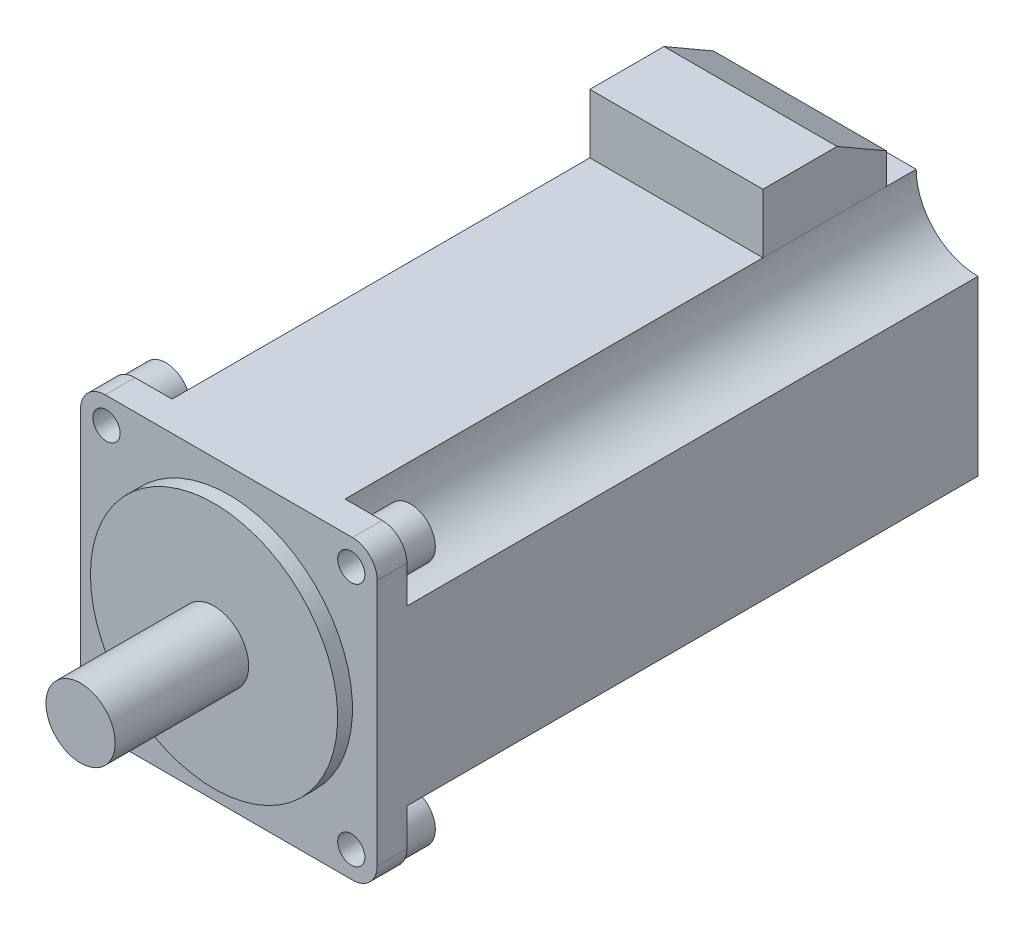
from build123d import *

# Parameters (mm, degrees)
SKETCH1_R                      = 7
BOSS_EXTRUDE1_DEPTH            = 30
SKETCH2_R                      = 25
BOSS_EXTRUDE2_DEPTH            = 3
SKETCH3_W                      = 60
SKETCH3_H                      = 60
BOSS_EXTRUDE3_DEPTH            = 6
BOSS_EXTRUDE4_DEPTH            = 115.5
SKETCH5_W                      = 35
SKETCH5_H                      = 25
BOSS_EXTRUDE5_DEPTH            = 12
CHAMFER1_SIZE                  = 10
CHAMFER1_SIZE2                 = 5.773502692
F_5_5_5_5_DIAMETER_HOLE1_D     = 5.5
F_5_5_5_5_DIAMETER_HOLE1_DEPTH = 20
F_5_5_5_5_DIAMETER_HOLE1_TIP   = 1.652366702
FILLET1_R                      = 5
SKETCH8_R                      = 5
BOSS_EXTRUDE6_DEPTH            = 6


with BuildPart() as part:
    # Sketch1 → Boss-Extrude1 (new body)
    with BuildSketch(Plane.XY):
        Circle(SKETCH1_R)
    extrude(amount=-BOSS_EXTRUDE1_DEPTH)

    # Sketch2 → Boss-Extrude2 (add)
    with BuildSketch(Plane(origin=(0, 0, -30), x_dir=(-1, 0, 0), z_dir=(0, 0, -1))):
        Circle(SKETCH2_R)
    extrude(amount=-BOSS_EXTRUDE2_DEPTH)

    # Sketch3 → Boss-Extrude3 (add)
    with BuildSketch(Plane(origin=(0, 0, -30), x_dir=(-1, 0, 0), z_dir=(0, 0, -1))):
        Rectangle(SKETCH3_W, SKETCH3_H)
    extrude(amount=BOSS_EXTRUDE3_DEPTH)

    # Sketch4 → Boss-Extrude4 (add)
    with BuildSketch(Plane(origin=(0, 0, -36), x_dir=(-1, 0, 0), z_dir=(0, 0, -1))):
        with BuildLine():
            Line((30, -17.5), (30, 17.5))
            ThreePointArc((30, 17.5), (21.161165235, 21.161165235), (17.5, 30))
            Line((17.5, 30), (-17.5, 30))
            ThreePointArc((-17.5, 30), (-21.161165235, 21.161165235), (-30, 17.5))
            Line((-30, 17.5), (-30, -17.5))
            ThreePointArc((-30, -17.5), (-21.161165235, -21.161165235), (-17.5, -30))
            Line((-17.5, -30), (17.5, -30))
            ThreePointArc((17.5, -30), (21.161165235, -21.161165235), (30, -17.5))
        make_face()
    extrude(amount=BOSS_EXTRUDE4_DEPTH)

    # Sketch5 → Boss-Extrude5 (add)
    with BuildSketch(Plane(origin=(0, 30, 0), x_dir=(1, 0, 0), z_dir=(0, 1, 0))):
        with Locations((0, 133)):
            Rectangle(SKETCH5_W, SKETCH5_H)
    extrude(amount=BOSS_EXTRUDE5_DEPTH)

    # Chamfer1
    chamfer1_edges = [part.edges().sort_by_distance(p)[0] for p in [
        (0, 42, -145.5),
    ]]
    chamfer1_side = [part.faces().sort_by_distance(p)[0] for p in [
        (0, 42, -133),
    ]]
    chamfer(chamfer1_edges, length=CHAMFER1_SIZE, length2=CHAMFER1_SIZE2, reference=chamfer1_side[0])

    # Ø5.5 (5.5) Diameter Hole1
    with Locations(Plane.XY.offset(-30)):
        with Locations((24.748737342, 24.748737342), (-24.748737342, 24.748737342), (24.748737342, -24.748737342), (-24.748737342, -24.748737342)):
            Hole(F_5_5_5_5_DIAMETER_HOLE1_D / 2, depth=F_5_5_5_5_DIAMETER_HOLE1_DEPTH)
            with Locations((0, 0, -(F_5_5_5_5_DIAMETER_HOLE1_DEPTH + F_5_5_5_5_DIAMETER_HOLE1_TIP / 2))):  # 118° drill point
                Cone(0, F_5_5_5_5_DIAMETER_HOLE1_D / 2, F_5_5_5_5_DIAMETER_HOLE1_TIP, mode=Mode.SUBTRACT)

    # Fillet1
    fillet1_edges = [part.edges().sort_by_distance(p)[0] for p in [
        (30, -30, -33),
        (-30, -30, -33),
        (-30, 30, -33),
        (30, 30, -33),
    ]]
    fillet(fillet1_edges, radius=FILLET1_R)

    # Sketch8 → Boss-Extrude6 (add)
    with BuildSketch(Plane(origin=(0, 0, -36), x_dir=(-1, 0, 0), z_dir=(0, 0, -1))):
        with Locations((-24.748737342, 24.748737342)):
            Circle(SKETCH8_R)
        with Locations((-24.748737342, -24.748737342)):
            Circle(SKETCH8_R)
        with Locations((24.748737342, -24.748737342)):
            Circle(SKETCH8_R)
        with Locations((24.748737342, 24.748737342)):
            Circle(SKETCH8_R)
    extrude(amount=BOSS_EXTRUDE6_DEPTH)


solid = part.part
